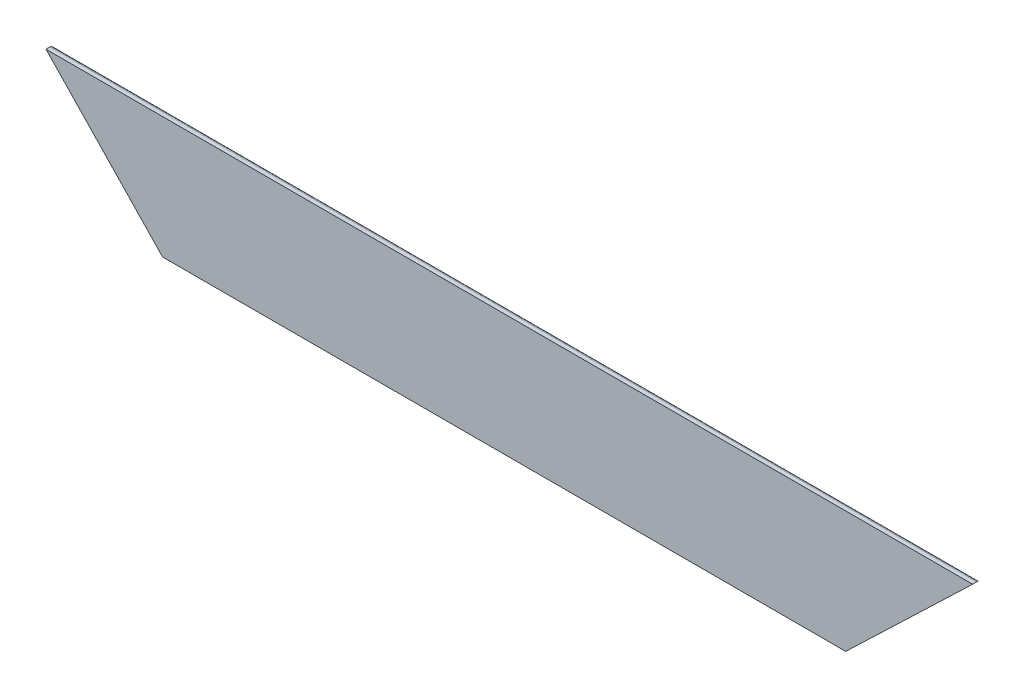
SolidWorks part; units mm, degrees
material "普通碳钢"
ref_plane "Front Plane" through (0, 0, 0) normal (0, 0, 1) x (1, 0, 0)
ref_plane "Top Plane" through (0, 0, 0) normal (0, 1, 0) x (1, 0, 0)
ref_plane "Right Plane" through (0, 0, 0) normal (1, 0, 0) x (0, 0, -1)
sketch "Sketch1" plane through (0, 0, 0) normal (1, 0, 0) x (0, 0, -1)
  line L1 (-44, 47.3) -> (-44, -32)
  line L2 (-32, -44) -> (47.3, -44)
  line L3 (50, -46.7) -> (50, -50)
  line L4 (50, -50) -> (-50, -50)
  line L5 (-50, -50) -> (-50, 50)
  line L6 (-50, 50) -> (-46.7, 50)
  arc A0 (-32, -44) -> (-44, -32) centre (-32, -32) cw
  arc A1 (-44, 47.3) -> (-46.7, 50) centre (-46.7, 47.3) ccw
  arc A2 (50, -46.7) -> (47.3, -44) centre (47.3, -46.7) ccw
  point P12 (0, -50)
  point P14 (-50, 0)
  dimension "D5" = 12
  dimension "D6" = 2.7
  dimension "D7" = 2.7
  dimension "D1" = 100
  dimension "D2" = 100
  dimension "D3" = 6
  dimension "D4" = 6
extrude "Extrude1" add sketch "Sketch1" along normal mid plane 1800
sketch "Sketch2" plane through (0, 0, 50) normal (0, 0, 1) x (1, 0, 0)
  line L0 (-900, 50) -> (-502.8764, 430.5166) construction
  line L1 (-502.8764, 430.5166) -> (-138.2724, 50) construction
  line L2 (-138.2724, 50) -> (-900, 50)
  line L5 (-900, 50) -> (-535.3959, -330.5166)
  line L6 (-535.3959, -330.5166) -> (-138.2724, 50)
  dimension "D1" = 550
  dimension "D2" = 527
extrude "Extrude5" cut sketch "Sketch2" against normal blind 100 flip side to cut
